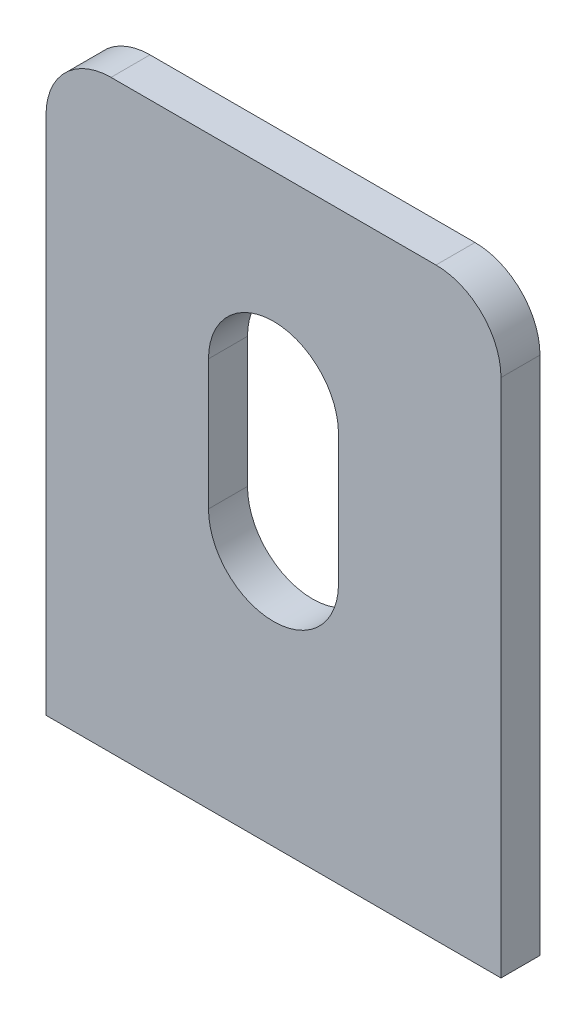
from build123d import *

# Parameters (mm, degrees)
BOSS_EXTRUDE1_DEPTH = 3


with BuildPart() as part:
    # Sketch1 → Boss-Extrude1 (new body)
    with BuildSketch(Plane.XY):
        with BuildLine():
            Line((0, 0), (35, 0))
            Line((35, 0), (35, 40))
            ThreePointArc((35, 40), (33.535533906, 43.535533906), (30, 45))
            Line((30, 45), (5, 45))
            ThreePointArc((5, 45), (1.464466094, 43.535533906), (0, 40))
            Line((0, 40), (0, 0))
        make_face()
        with BuildLine():
            Line((12.5, 30), (12.5, 20))
            ThreePointArc((12.5, 20), (17.5, 15), (22.5, 20))
            Line((22.5, 20), (22.5, 30))
            ThreePointArc((22.5, 30), (17.5, 35), (12.5, 30))
        make_face(mode=Mode.SUBTRACT)
    extrude(amount=BOSS_EXTRUDE1_DEPTH)


solid = part.part
